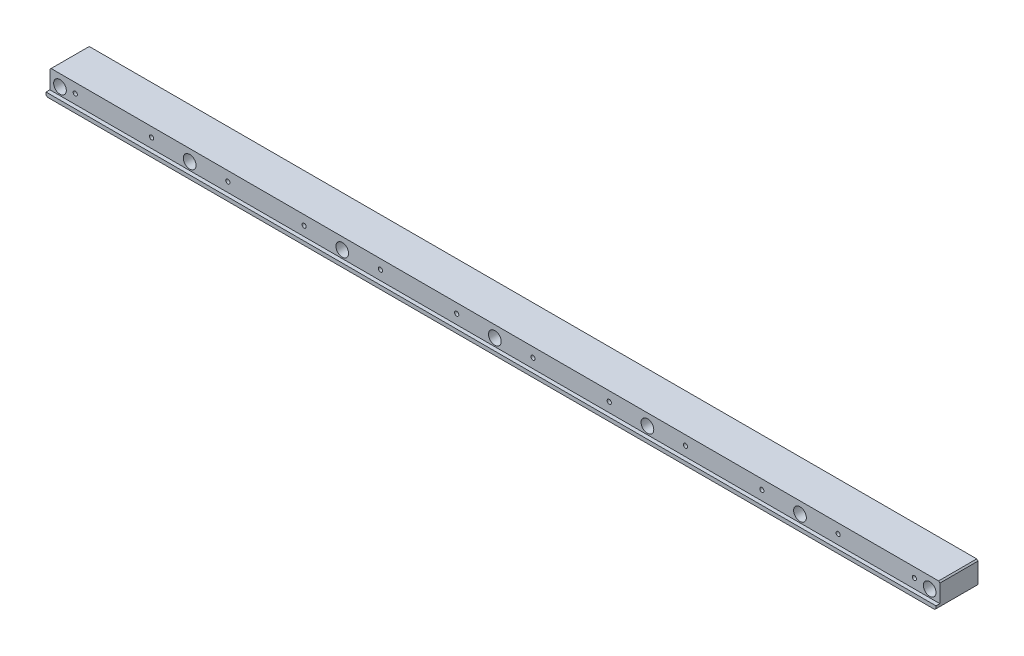
SolidWorks part; units mm, degrees
material "AL6061"
ref_plane "Front Plane" through (0, 0, 0) normal (0, 0, 1) x (1, 0, 0)
ref_plane "Top Plane" through (0, 0, 0) normal (0, 1, 0) x (1, 0, 0)
ref_plane "Right Plane" through (0, 0, 0) normal (1, 0, 0) x (0, 0, -1)
sketch "Sketch1" plane through (0, 0, 0) normal (0, 0, 1) x (1, 0, 0)
  line L1 (-350, 9) -> (350, 9)
  line L2 (-350, 9) -> (-350, -9)
  line L3 (-350, -9) -> (350, -9)
  line L4 (350, 9) -> (350, -9)
  line L5 (-350, 9) -> (350, -9) construction
  line L6 (-350, -9) -> (350, 9) construction
  point P0 (0, 0)
  dimension "D1" = 18
  dimension "D2" = 700
extrude "Boss-Extrude1" add sketch "Sketch1" along normal mid plane 33
sketch "Sketch4" plane through (0, 0, 16.5) normal (0, 0, 1) x (1, 0, 0)
  line L1 (-350, 9) -> (350, 9)
  line L2 (-350, 9) -> (-350, -6)
  line L3 (-350, -6) -> (350, -6)
  line L4 (350, 9) -> (350, -6)
  line L5 (-350, 9) -> (350, -6) construction
  line L6 (-350, -6) -> (350, 9) construction
  line L7 (-350, -9) -> (350, -9) construction
  line L8 (-350, 9) -> (-350, -9) construction
  line L9 (350, -9) -> (350, 9) construction
  line L10 (350, 9) -> (-350, 9) construction
  point P0 (0, 1.5)
  dimension "D1" = 3
extrude "Cut-Extrude1" cut sketch "Sketch4" against normal blind 3
hole_wizard "M4 Tapped Hole1" positions "Sketch5" profile "Sketch6" tap size "M4" standard "ISO"
sketch "Sketch5" plane through (0, 0, 13.5) normal (0, 0, 1) x (1, 0, 0)
  point P0 (330, 1.5)
  point P3 (270, 1.5)
  point P6 (210, 1.5)
  point P9 (150, 1.5)
  point P12 (90, 1.5)
  point P15 (30, 1.5)
  point P18 (-30, 1.5)
  point P21 (-90, 1.5)
  point P24 (-150, 1.5)
  point P27 (-330, 1.5)
  point P31 (-210, 1.5)
  point P34 (-270, 1.5)
sketch "Sketch6" plane through (330, 1.5, 13.5) normal (1, 0, 0) x (0, -1, 0)
  line L0 (0, 0) -> (0, 16.4914)
  line L1 (0, 16.4914) -> (1.65, 15.5)
  line L2 (1.65, 15.5) -> (1.65, 0)
  line L5 (1.65, 0) -> (0, 0)
  line L10 (0, 16.4914) -> (-1.65, 15.5) construction
  line L11 (0, -6.35) -> (0, 107.95) construction
  dimension "螺纹孔钻头直径" = 3.3
  dimension "螺纹孔钻头深度" = 15.5
  dimension "导头角度" = 118
cosmetic thread "Cosmetic thread 1" parameters "D1"=12, "D2"=4
cosmetic thread "Cosmetic thread 2" parameters "D1"=12, "D2"=4
cosmetic thread "Cosmetic thread 3" parameters "D1"=12, "D2"=4
cosmetic thread "Cosmetic thread 4" parameters "D1"=12, "D2"=4
cosmetic thread "Cosmetic thread 5" parameters "D1"=12, "D2"=4
cosmetic thread "Cosmetic thread 6" parameters "D1"=12, "D2"=4
cosmetic thread "Cosmetic thread 7" parameters "D1"=12, "D2"=4
cosmetic thread "Cosmetic thread 8" parameters "D1"=12, "D2"=4
cosmetic thread "Cosmetic thread 9" parameters "D1"=12, "D2"=4
cosmetic thread "Cosmetic thread 10" parameters "D1"=12, "D2"=4
cosmetic thread "Cosmetic thread 11" parameters "D1"=12, "D2"=4
cosmetic thread "Cosmetic thread 12" parameters "D1"=12, "D2"=4
hole_wizard "CBORE for M5 Hex Socket Head Cap Screw1" positions "Sketch7" profile "Sketch8" counterbore size "M5" standard "ISO" end condition through all
sketch "Sketch7" plane through (0, 0, 16.5) normal (0, 0, 1) x (1, 0, 0)
  line L0 (0, 0) -> (0, 46.862) construction
  line L3 (-350, 9) -> (-350, -6) construction
  circle A0 centre (-210, 1.5) radius 1.65 construction
  circle A1 centre (-90, 1.5) radius 1.65 construction
  point P0 (-342, 0)
  point P4 (-240, 0)
  point P6 (-120, 0)
  point P8 (0, 0)
  point P10 (120, 0)
  point P12 (240, 0)
  point P14 (342, 0)
  dimension "D3" = 30
  dimension "D1" = 8
  dimension "D2" = 30
sketch "Sketch8" plane through (-342, 0, 16.5) normal (1, 0, 0) x (0, -1, 0)
  line L0 (0, 0) -> (0, 33)
  line L1 (0, 33) -> (2.75, 33)
  line L3 (2.75, 33) -> (2.75, 18)
  line L4 (2.75, 18) -> (5, 18)
  line L5 (5, 18) -> (5, 0)
  line L7 (5, 0) -> (0, 0)
  line L11 (0, -6.35) -> (0, 107.95) construction
  dimension "通孔孔直径" = 5.5
  dimension "通孔孔深度" = 33
  dimension "柱形沉头孔直径" = 10
  dimension "柱形沉头孔深度" = 18
hole_wizard "Size mm dowel hole 1" positions "Sketch10" profile "Sketch11" hole size "Ø8.0" standard "ISO"
sketch "Sketch10" plane through (0, 0, -16.5) normal (0, 0, -1) x (-1, 0, 0)
  line L1 (0, 0) -> (0, 23.6902) construction
  circle A0 centre (330, 1.5) radius 1.65 construction
  point P0 (-300, 0)
  point P2 (300, 0)
  dimension "D1" = 30
sketch "Sketch11" plane through (300, 0, -16.5) normal (1, 0, 0) x (0, 1, 0)
  line L0 (0, 0) -> (0, 13.4034)
  line L1 (0, 13.4034) -> (4, 11)
  line L2 (4, 11) -> (4, 0)
  line L5 (4, 0) -> (0, 0)
  line L10 (0, 13.4034) -> (-4, 11) construction
  line L11 (0, -6.35) -> (0, 107.95) construction
  dimension "孔直径" = 8
  dimension "孔深度" = 11
  dimension "导头角度" = 118
chamfer "Chamfer1" distance 1 angle 45 4 edges at (350, 9, -1.5) (350, -9, 0) (-350, -9, 0) (-350, 9, -1.5)
